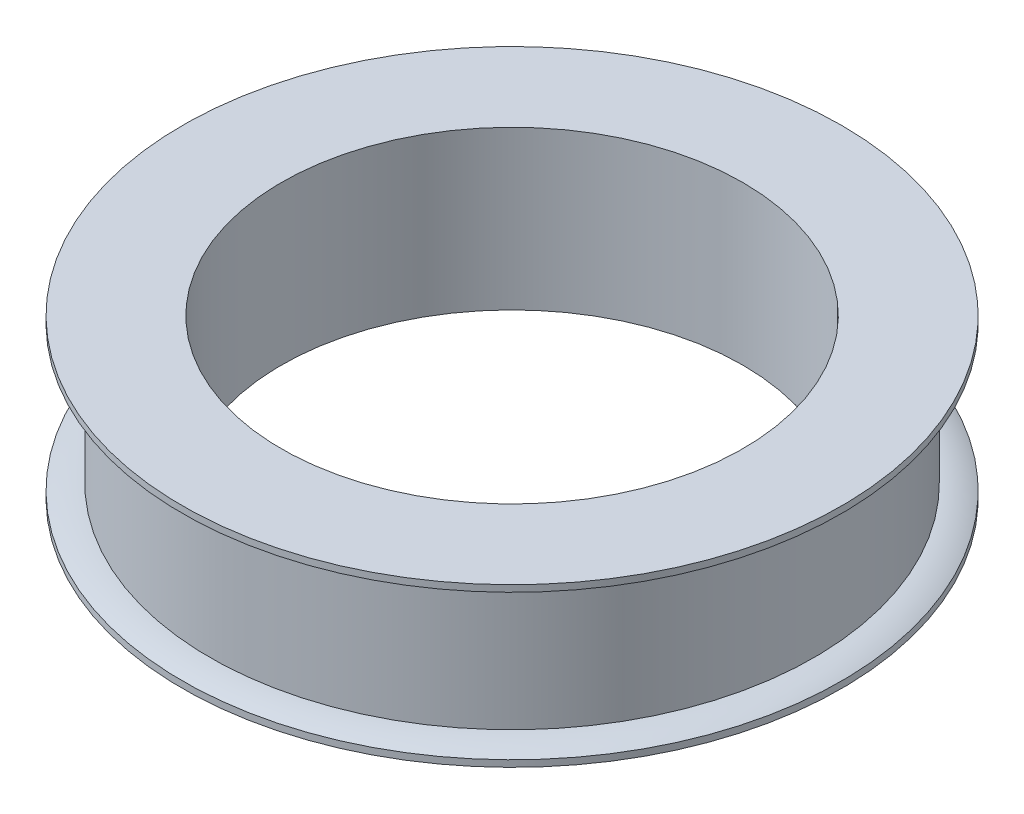
from build123d import *


with BuildPart() as part:
    # Sketch1 → Revolve1 (revolve)
    with BuildSketch(Plane.XY, mode=Mode.PRIVATE) as revolve1_sk:
        Polygon((22.92, -5), (22.92, 5), (20, 5), (20, 6), (17.5, 6), (17.5, -6), (20, -6), (20, -5), align=None)
    revolve(revolve1_sk.sketch.rotate(Axis((0, 0, 0), (0, 1, 0)), 90), axis=Axis((0, 0, 0), (0, 1, 0)))

    # Sketch2 → Revolve2 (revolve)
    with BuildSketch(Plane.XY, mode=Mode.PRIVATE) as revolve2_sk:
        with BuildLine():
            Line((20, 5), (22.92, 5))
            ThreePointArc((22.92, 5), (23.9870538, 5.137456193), (25, 5.5))
            Line((25, 5.5), (25, 6))
            Line((25, 6), (20, 6))
            Line((20, 6), (20, 5))
        make_face()
        with BuildLine():
            Line((25, -5.5), (25, -6))
            Line((25, -6), (20, -6))
            Line((20, -6), (20, -5))
            Line((20, -5), (22.92, -5))
            ThreePointArc((22.92, -5), (23.9870538, -5.137456193), (25, -5.5))
        make_face()
    revolve(revolve2_sk.sketch.rotate(Axis((0, 0, 0), (0, 1, 0)), 90), axis=Axis((0, 0, 0), (0, 1, 0)))


solid = part.part
